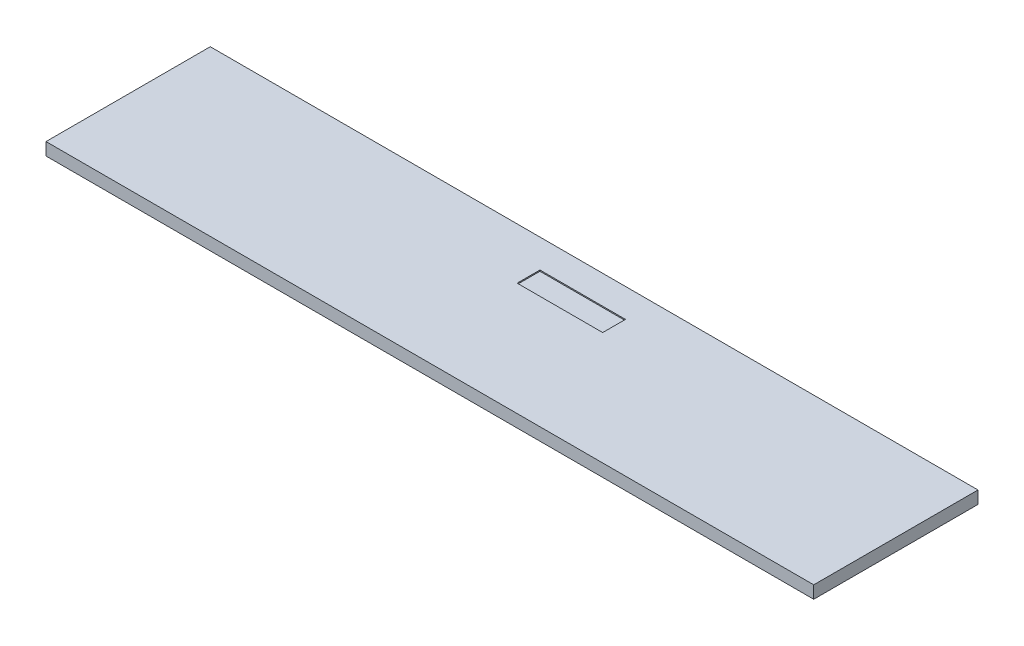
SolidWorks part; units mm, degrees
ref_plane "前视" through (0, 0, 0) normal (0, 0, 1) x (1, 0, 0)
ref_plane "上视" through (0, 0, 0) normal (0, 1, 0) x (1, 0, 0)
ref_plane "右视" through (0, 0, 0) normal (1, 0, 0) x (0, 0, -1)
sketch "草图1" plane through (0, 0, 0) normal (0, 1, 0) x (1, 0, 0)
  line L0 (0, 0) -> (0, 42.2558) construction
  line L1 (-673, 144) -> (673, 144)
  line L2 (-673, 144) -> (-673, -144)
  line L3 (-673, -144) -> (673, -144)
  line L4 (673, 144) -> (673, -144)
  line L5 (0, 0) -> (74.6519, 0) construction
  dimension "D1" = 288
  dimension "D2" = 1346
  dimension "D3" = 673
  dimension "D4" = 144
extrude "凸台-拉伸1" add sketch "草图1" against normal blind 20
shell "抽壳1" thickness 2
sketch "草图2" plane through (0, -20, 0) normal (0, -1, 0) x (1, 0, 0)
  line L0 (0, 0) -> (0, -281.5139) construction
  line L1 (-673, -144) -> (673, -144)
  line L2 (-673, -144) -> (-673, 144)
  line L3 (-673, 144) -> (673, 144)
  line L4 (673, -144) -> (673, 144)
  line L5 (0, 0) -> (604.9925, 0) construction
  line L6 (-673, -144) -> (-673, 144) construction
  line L7 (673, 144) -> (673, -144) construction
  dimension "D2" = 288
  dimension "D4" = 144
extrude "凸台-拉伸2" add sketch "草图2" along normal blind 2
sketch "草图4" plane through (0, 0, 0) normal (0, 1, 0) x (1, 0, 0)
  line L0 (673, 144) -> (-673, 144) construction
  line L1 (-45, 94) -> (105, 94)
  line L2 (-45, 94) -> (-45, 54)
  line L3 (-45, 54) -> (105, 54)
  line L4 (105, 94) -> (105, 54)
  line L5 (-673, 144) -> (-673, -144) construction
  dimension "D1" = 150
  dimension "D2" = 40
  dimension "D3" = 50
  dimension "D4" = 628
extrude "切除-拉伸1" cut sketch "草图4" against normal blind 2
